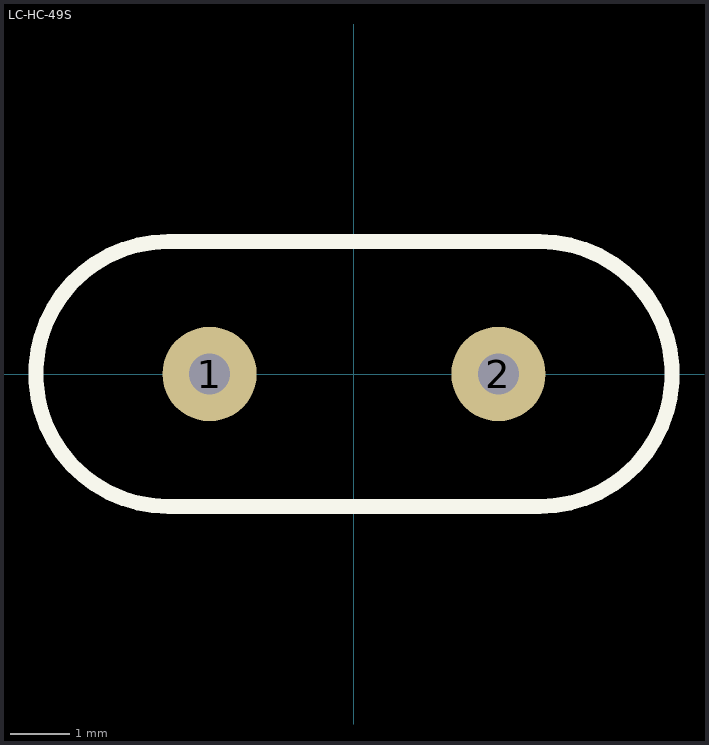
[diagram p0: the footprint, top view; thin cyan lines are the x and y axes]
# Altium footprint library MISC89328-6.PcbLib: 1 footprints
Each footprint in its own frame and in the unit in brackets; x right, y up, seen from the top. Pads: shape width x height; smd on the part's side, far side on the other; paste and mask are expansions set on the pad; w line width, h text height; cw(c..) or ccw(c..) is an arc to the next point about the centre after c.

## LC-HC-49S [mm]
pads (2):
  round 1.6 hole 0.7: 1(-2.45,0) 2(2.45,0)
Top Overlay:
  lines w0.254: -3.15,-2.248 cw(c-3.15,0) -3.15,2.248 3.15,2.248 cw(c3.15,0) 3.15,-2.248 -3.15,-2.248
3D body "hc-49s_n.stp": height 3.6, standoff -2.9, extent -5.388,-2.27 5.412,2.23